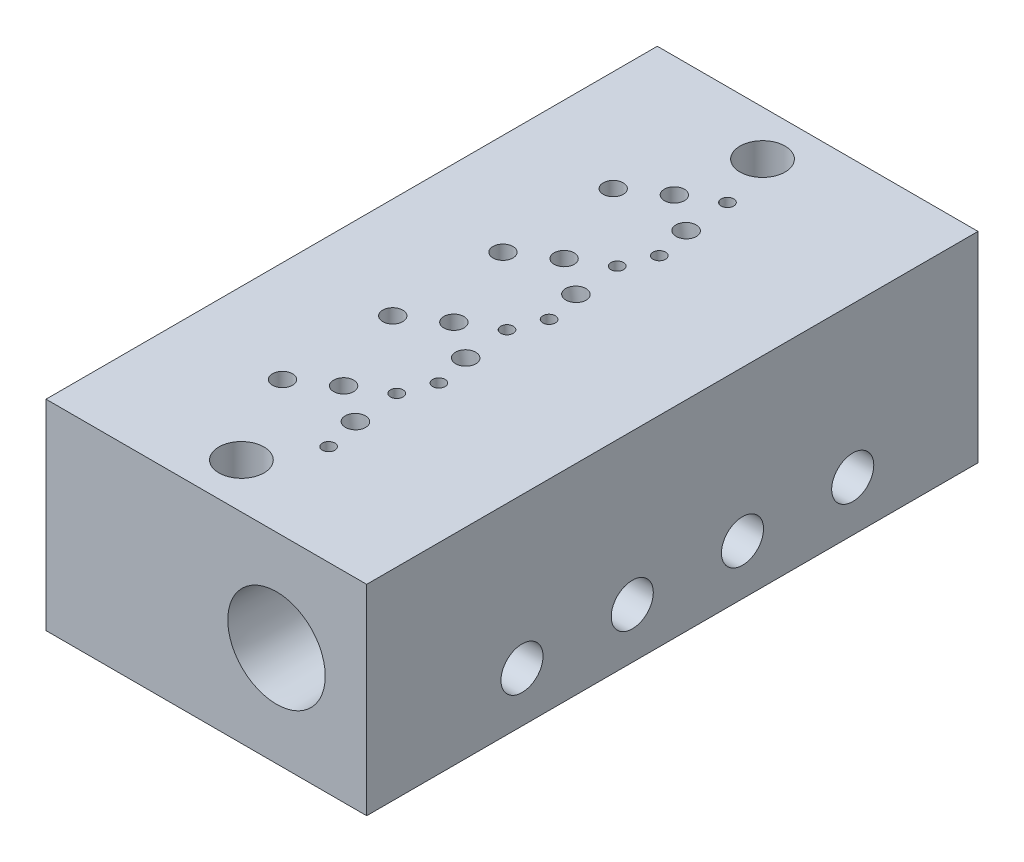
SolidWorks part; units mm, degrees
ref_plane "Front Plane" through (0, 0, 0) normal (0, 0, 1) x (1, 0, 0)
ref_plane "Top Plane" through (0, 0, 0) normal (0, 1, 0) x (1, 0, 0)
ref_plane "Right Plane" through (0, 0, 0) normal (1, 0, 0) x (0, 0, -1)
sketch "Sketch1" plane through (0, 0, 0) normal (0, 0, 1) x (1, 0, 0)
  line L0 (-32, 0) -> (0, 0)
  line L1 (0, 0) -> (0, -20)
  line L2 (0, -20) -> (-32, -20)
  line L7 (-32, -20) -> (-32, 0)
  dimension "D1" = 32
  dimension "D2" = 20
extrude "Boss-Extrude1" add sketch "Sketch1" against normal blind 61
hole_wizard "1/8 Rc Tapped Hole2" positions "Sketch6" profile "Sketch5" size "1/8" standard "Iso"
sketch "Sketch6" plane through (16.8214, 4.3225, 0) normal (0, 0, -1) x (-1, 0, 0)
  line L0 (16.8214, -24.3225) -> (16.8214, -4.3225) construction
  line L1 (16.8214, -4.3225) -> (48.8214, -4.3225) construction
  point P0 (25.8214, -14.3225)
  dimension "D1" = 9
  dimension "D2" = 10
sketch "Sketch5" plane through (-9, -10, 0) normal (1, 0, 0) x (0, -1, 0)
  line L0 (0, 0) -> (0, 10.8734)
  line L1 (3.95, 8.5) -> (0, 10.8734)
  line L2 (-3.95, 8.5) -> (0, 10.8734) construction
  line L3 (3.95, 8.5) -> (3.95, 7.4)
  line L4 (3.95, 7.4) -> (4.633, 7.4)
  line L5 (4.633, 7.4) -> (4.864, 0)
  line L6 (-4.633, 7.4) -> (-4.864, 0) construction
  line L7 (4.864, 0) -> (0, 0)
  line L8 (0, -6.35) -> (0, 107.95) construction
  line L11 (-3.95, 7.4) -> (-4.633, 7.4) construction
  dimension "螺纹孔钻头直径" = 7.9
  dimension "螺纹孔钻头深度" = 8.5
  dimension "螺纹直径" = 9.728
  dimension "螺纹角度" = 3.576
  dimension "螺纹深度" = 7.4
  dimension "导头角度" = 118
sketch "Sketch8" plane through (0, 0, 0) normal (0, 0, 1) x (1, 0, 0)
  line L0 (-8, -8) -> (-11.9641, -8) construction
  line L1 (-8, -8) -> (-8, -12) construction
  line L2 (-11.9641, -12) -> (-8, -12) construction
  line L3 (0, -20) -> (0, 0) construction
  line L4 (-8.5, -10) -> (-23.4984, -10) construction
  arc A0 (-11.9641, -12) -> (-11.9641, -8) centre (-8.5, -10) cw construction
  circle A1 centre (-10.5, -10) radius 2.25
  circle A3 centre (-9, -10) radius 3.95 construction
  point P5 (-8, -10)
  dimension "D1" = 4
  dimension "D6" = 4.5
  dimension "D7" = 1.5
  dimension "D2" = 8
  dimension "D3" = 8.5
  dimension "D4" = 10
  dimension "D5" = 4
extrude "Cut-Extrude3" cut sketch "Sketch8" against normal offset from surface (53 mm away) 8 up to face at (-16, -10, -61)
sketch "Sketch9" plane through (0, 0, 0) normal (0, 1, 0) x (1, 0, 0)
  line L0 (0, 0) -> (-32, 0) construction
  line L2 (0, 61) -> (0, 0) construction
  circle A0 centre (-21.9, 13.5) radius 1
  dimension "D1" = 2
  dimension "D3" = 21.9
  dimension "D2" = 13.5
extrude "Cut-Extrude4" cut sketch "Sketch9" against normal blind 10
hole_wizard "M5 Tapped Hole1" positions "Sketch12" profile "Sketch11" tap size "M5" standard "Gb"
sketch "Sketch12" plane through (0, 0, 0) normal (1, 0, 0) x (0, 0, -1)
  line L0 (39, 0) -> (0, 0) construction
  line L1 (0, -20) -> (0, 0) construction
  point P0 (15.5, -5)
  dimension "D1" = 5
  dimension "D2" = 15.5
sketch "Sketch11" plane through (0, -5, -15.5) normal (0, 1, 0) x (0, 0, -1)
  line L0 (0, 0) -> (0, 12.7618)
  line L1 (0, 12.7618) -> (2.1, 11.5)
  line L2 (2.1, 11.5) -> (2.1, 0)
  line L5 (2.1, 0) -> (0, 0)
  line L10 (0, 12.7618) -> (-2.1, 11.5) construction
  line L11 (0, -6.35) -> (0, 107.95) construction
  dimension "螺纹孔钻头直径" = 4.2
  dimension "螺纹孔钻头深度" = 11.5
  dimension "导头角度" = 118
cosmetic thread "Cosmetic thread 1" [suppressed] parameters "D1"=5, "D2"=5
hole_wizard "M5 Tapped Hole2" positions "Sketch14" profile "Sketch13" tap size "M5" standard "Gb"
sketch "Sketch14" plane through (0, 0, 0) normal (1, 0, 0) x (0, 0, -1)
  line L0 (0, -20) -> (0, 0) construction
  line L1 (61, 0) -> (0, 0) construction
  point P0 (15.5, -15)
  dimension "D1" = 15
  dimension "D2" = 15.5
sketch "Sketch13" plane through (0, -15, -15.5) normal (0, 1, 0) x (0, 0, -1)
  line L0 (0, 0) -> (0, 21.2618)
  line L1 (0, 21.2618) -> (2.1, 20)
  line L2 (2.1, 20) -> (2.1, 0)
  line L5 (2.1, 0) -> (0, 0)
  line L10 (0, 21.2618) -> (-2.1, 20) construction
  line L11 (0, -6.35) -> (0, 107.95) construction
  dimension "螺纹孔钻头直径" = 4.2
  dimension "螺纹孔钻头深度" = 20
  dimension "导头角度" = 118
cosmetic thread "Cosmetic thread 2" parameters "D1"=5, "D2"=5
ref_plane "Plane1" through (0, 0, 0) normal (-0.1736, 0.9848, 0) x (0.9848, 0.1736, 0)
ref_plane "Plane2" through (1.5628, -8.8633, 0) normal (-0.1736, 0.9848, 0) x (0.9848, 0.1736, 0)
sketch "Sketch16" plane through (1.5628, -8.8633, 0) normal (-0.1736, 0.9848, 0) x (0.9848, 0.1736, 0)
  line L0 (0, 0) -> (-31.5138, 0) construction
  line L1 (0, 61) -> (0, 0) construction
  circle A0 centre (-14.4, 13.5) radius 1
  dimension "D1" = 2
  dimension "D2" = 13.5
  dimension "D3" = 14.4
extrude "Cut-Extrude5" cut sketch "Sketch16" along normal up to surface (11.7154 mm away)
sketch "Sketch17" plane through (0, 0, 0) normal (0, 1, 0) x (1, 0, 0)
  line L0 (0, 61) -> (0, 0) construction
  line L2 (0, 0) -> (-32, 0) construction
  circle A0 centre (-18.3, 16) radius 1
  dimension "D1" = 2
  dimension "D2" = 18.3
  dimension "D3" = 16
extrude "Cut-Extrude6" cut sketch "Sketch17" against normal blind 15
sketch "Sketch18" plane through (0, 0, 0) normal (0, 1, 0) x (1, 0, 0)
  line L0 (0, 0) -> (-32, 0) construction
  line L1 (0, 61) -> (0, 0) construction
  circle A0 centre (-11, 16) radius 1
  dimension "D1" = 2
  dimension "D2" = 16
  dimension "D3" = 11
extrude "Cut-Extrude7" [suppressed] cut sketch "Sketch18" against normal blind 5
hole_wizard "M1.6 Tapped Hole1" positions "Sketch20" profile "Sketch19" tap size "M1.6" standard "Gb"
sketch "Sketch20" plane through (0, 0, 0) normal (0, 1, 0) x (1, 0, 0)
  line L0 (0, 0) -> (-32, 0) construction
  line L2 (0, 61) -> (0, 0) construction
  point P0 (-13.8, 10)
  point P2 (-15, 18)
  dimension "D1" = 10
  dimension "D2" = 13.8
  dimension "D3" = 1.2
  dimension "D4" = 8
sketch "Sketch19" plane through (-13.8, 0, -10) normal (1, 0, 0) x (0, 0, 1)
  line L0 (0, 0) -> (0, 4.6255)
  line L1 (0, 4.6255) -> (0.625, 4.25)
  line L2 (0.625, 4.25) -> (0.625, 0)
  line L5 (0.625, 0) -> (0, 0)
  line L10 (0, 4.6255) -> (-0.625, 4.25) construction
  line L11 (0, -6.35) -> (0, 107.95) construction
  dimension "螺纹孔钻头直径" = 1.25
  dimension "螺纹孔钻头深度" = 4.25
  dimension "导头角度" = 118
cosmetic thread "Cosmetic thread 3" parameters "D1"=3, "D2"=1.6
cosmetic thread "Cosmetic thread 4" parameters "D1"=3, "D2"=1.6
hole_wizard "Ø4.5 (4.5) Diameter Hole1" positions "Sketch22" profile "Sketch21" hole size "Ø4.5" standard "Gb" end condition through all
sketch "Sketch22" plane through (0, 0, 0) normal (0, 1, 0) x (1, 0, 0)
  line L0 (-17, 56.5) -> (-17, 4.5) construction
  line L2 (0, 0) -> (-32, 0) construction
  line L3 (0, 61) -> (0, 0) construction
  point P0 (-17, 4.5)
  point P2 (-17, 56.5)
  dimension "D1" = 52
  dimension "D2" = 4.5
  dimension "D3" = 17
sketch "Sketch21" plane through (-17, 0, -4.5) normal (1, 0, 0) x (0, 0, 1)
  line L0 (0, 0) -> (0, 20)
  line L1 (0, 20) -> (2.25, 20)
  line L2 (2.25, 20) -> (2.25, 0)
  line L5 (2.25, 0) -> (0, 0)
  line L11 (0, -6.35) -> (0, 107.95) construction
  dimension "通孔孔直径" = 4.5
  dimension "通孔孔深度" = 20
ref_axis "Axis1" through (-14.5423, -0.4528, -13.5) along (0.1736, -0.9848, 0)
ref_plane "Plane3" through (0, 0, -13.5) normal (0, 0, 1) x (1, 0, 0)
sketch "Sketch24" plane through (0, 0, -13.5) normal (0, 0, 1) x (1, 0, 0)
  line L0 (-14.5423, -0.4528) -> (-12.6797, -11.0159) construction
  line L1 (-12.6184, -11.3638) -> (-11.6336, -11.1902)
  line L2 (-11.6336, -11.1902) -> (-12.5141, -11.9555)
  line L3 (-12.5141, -11.9555) -> (-12.6184, -11.3638)
  line L5 (-12.3275, -11.3125) -> (-13.6032, -11.5375) construction
  dimension "D1" = 59
  dimension "D2" = 1
revolve "Cut-Revolve1" cut sketch "Sketch24" angle 360 about axis through (-14.5423, -0.4528, -13.5) along (0.1736, -0.9848, 0)
hole_wizard "M5 Tapped Hole3" positions "Sketch26" profile "Sketch25" tap size "M5" standard "Gb"
sketch "Sketch26" plane through (-32, 0, 0) normal (-1, 0, 0) x (0, 0, 1)
  line L0 (-61, 0) -> (0, 0) construction
  line L1 (0, 0) -> (0, -20) construction
  point P0 (-13.5, -10)
  dimension "D1" = 10
  dimension "D2" = 13.5
sketch "Sketch25" plane through (-32, -10, -13.5) normal (0, 1, 0) x (0, 0, 1)
  line L0 (0, 0) -> (0, 12.7618)
  line L1 (0, 12.7618) -> (2.1, 11.5)
  line L2 (2.1, 11.5) -> (2.1, 0)
  line L5 (2.1, 0) -> (0, 0)
  line L10 (0, 12.7618) -> (-2.1, 11.5) construction
  line L11 (0, -6.35) -> (0, 107.95) construction
  dimension "螺纹孔钻头直径" = 4.2
  dimension "螺纹孔钻头深度" = 11.5
  dimension "导头角度" = 118
cosmetic thread "Cosmetic thread 5" parameters "D1"=5, "D2"=5
pattern_linear "LPattern1" count 4 spacing 11 along (0, 0, -1) of "Cut-Extrude4", "Cut-Extrude5", "M1.6 Tapped Hole1", "Cut-Revolve1", "Cut-Extrude6", "M5 Tapped Hole2", "M5 Tapped Hole3"
